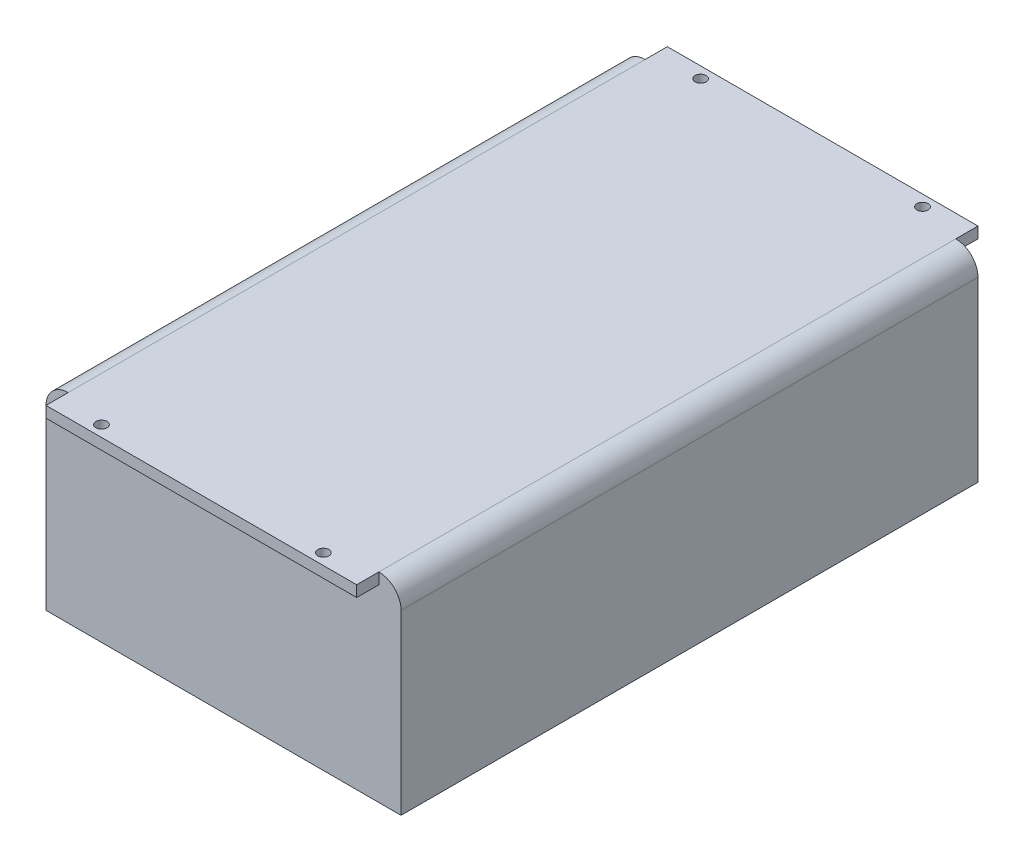
SolidWorks part; units mm, degrees
ref_plane "Front Plane" through (0, 0, 0) normal (0, 0, 1) x (1, 0, 0)
ref_plane "Top Plane" through (0, 0, 0) normal (0, 1, 0) x (1, 0, 0)
ref_plane "Right Plane" through (0, 0, 0) normal (1, 0, 0) x (0, 0, -1)
sketch "Sketch1" plane through (0, 0, 0) normal (0, 0, 1) x (1, 0, 0)
  line L1 (0, 0) -> (160, 0)
  line L2 (0, 0) -> (0, 90)
  line L3 (0, 90) -> (160, 90)
  line L4 (160, 0) -> (160, 90)
  dimension "D1" = 160
  dimension "D2" = 90
extrude "Boss-Extrude1" add sketch "Sketch1" along normal blind 260
fillet "Fillet2" radius 10 2 edges at (160, 90, 130) (0, 90, 130)
shell "Shell1" thickness 3
sketch "Sketch2" plane through (0, 87, 0) normal (0, -1, 0) x (-1, 0, 0)
  line L1 (-35, -88.2) -> (-137.87, -88.2) construction
  line L2 (-35, -88.2) -> (-35, -12) construction
  line L3 (-35, -12) -> (-137.87, -12) construction
  line L4 (-137.87, -88.2) -> (-137.87, -12) construction
  line L5 (-150, -3) -> (-10, -3) construction
  line L6 (-10, -3) -> (-10, -257) construction
  circle A0 centre (-35, -88.2) radius 2
  circle A1 centre (-35, -88.2) radius 5
  circle A2 centre (-35, -12) radius 5
  circle A3 centre (-35, -12) radius 2
  circle A4 centre (-137.87, -12) radius 5
  circle A5 centre (-137.87, -12) radius 2
  circle A6 centre (-137.87, -88.2) radius 5
  circle A7 centre (-137.87, -88.2) radius 2
  dimension "D4" = 4
  dimension "D5" = 10
  dimension "D6" = 4
  dimension "D7" = 4
  dimension "D8" = 4
  dimension "D9" = 10
  dimension "D10" = 10
  dimension "D11" = 10
  dimension "D1" = 102.87
  dimension "D2" = 76.2
  dimension "D3" = 9
  dimension "D12" = 25
extrude "Boss-Extrude2" add sketch "Sketch2" along normal blind 50
sketch "Sketch3" plane through (0, 87, 0) normal (0, -1, 0) x (-1, 0, 0)
  line L1 (-20, -114) -> (-140, -114) construction
  line L2 (-20, -114) -> (-20, -250) construction
  line L3 (-20, -250) -> (-140, -250) construction
  line L4 (-140, -114) -> (-140, -250) construction
  line L6 (0, -260) -> (-160, -260) construction
  circle A0 centre (-20, -114) radius 6
  circle A1 centre (-20, -114) radius 2
  circle A2 centre (-20, -250) radius 2
  circle A3 centre (-20, -250) radius 6
  circle A4 centre (-140, -114) radius 2
  circle A5 centre (-140, -114) radius 6
  circle A6 centre (-140, -250) radius 2
  circle A7 centre (-140, -250) radius 6
  dimension "D5" = 4
  dimension "D6" = 12
  dimension "D7" = 12
  dimension "D8" = 4
  dimension "D9" = 4
  dimension "D10" = 12
  dimension "D11" = 4
  dimension "D12" = 12
  dimension "D2" = 120
  dimension "D1" = 136
  dimension "D4" = 10
extrude "Boss-Extrude3" add sketch "Sketch3" along normal blind 6
sketch "Sketch4" plane through (0, 0, 0) normal (0, 0, -1) x (-1, 0, 0)
  line L1 (-10, 90) -> (-150, 90)
  line L2 (-10, 90) -> (-10, 85)
  line L3 (-10, 85) -> (-150, 85)
  line L4 (-150, 90) -> (-150, 85)
  dimension "D1" = 5
extrude "Boss-Extrude4" add sketch "Sketch4" along normal blind 10
sketch "Sketch5" plane through (0, 0, 260) normal (0, 0, 1) x (1, 0, 0)
  line L1 (150, 90) -> (10, 90)
  line L2 (150, 90) -> (150, 85)
  line L3 (150, 85) -> (10, 85)
  line L4 (10, 90) -> (10, 85)
  dimension "D1" = 5
extrude "Boss-Extrude5" add sketch "Sketch5" along normal blind 10
sketch "Sketch6" plane through (0, 85, 0) normal (0, -1, 0) x (-1, 0, 0)
  line L0 (-10, -270) -> (-150, -270) construction
  line L1 (-150, -270) -> (-150, -260) construction
  line L2 (-10, -270) -> (-10, -260) construction
  line L3 (-150, 10) -> (-10, 10) construction
  line L4 (-10, 10) -> (-10, 0) construction
  line L5 (-150, 10) -> (-150, 0) construction
  circle A0 centre (-130, -265) radius 2.5
  circle A1 centre (-30, -265) radius 2.5
  circle A2 centre (-130, 5) radius 2.5
  circle A3 centre (-30, 5) radius 2.5
  dimension "D1" = 5
  dimension "D2" = 5
  dimension "D3" = 5
  dimension "D4" = 5
  dimension "D5" = 5
  dimension "D6" = 5
  dimension "D7" = 20
  dimension "D8" = 20
  dimension "D9" = 5
  dimension "D10" = 20
  dimension "D11" = 20
  dimension "D12" = 5
extrude "Cut-Extrude1" cut sketch "Sketch6" against normal through all
